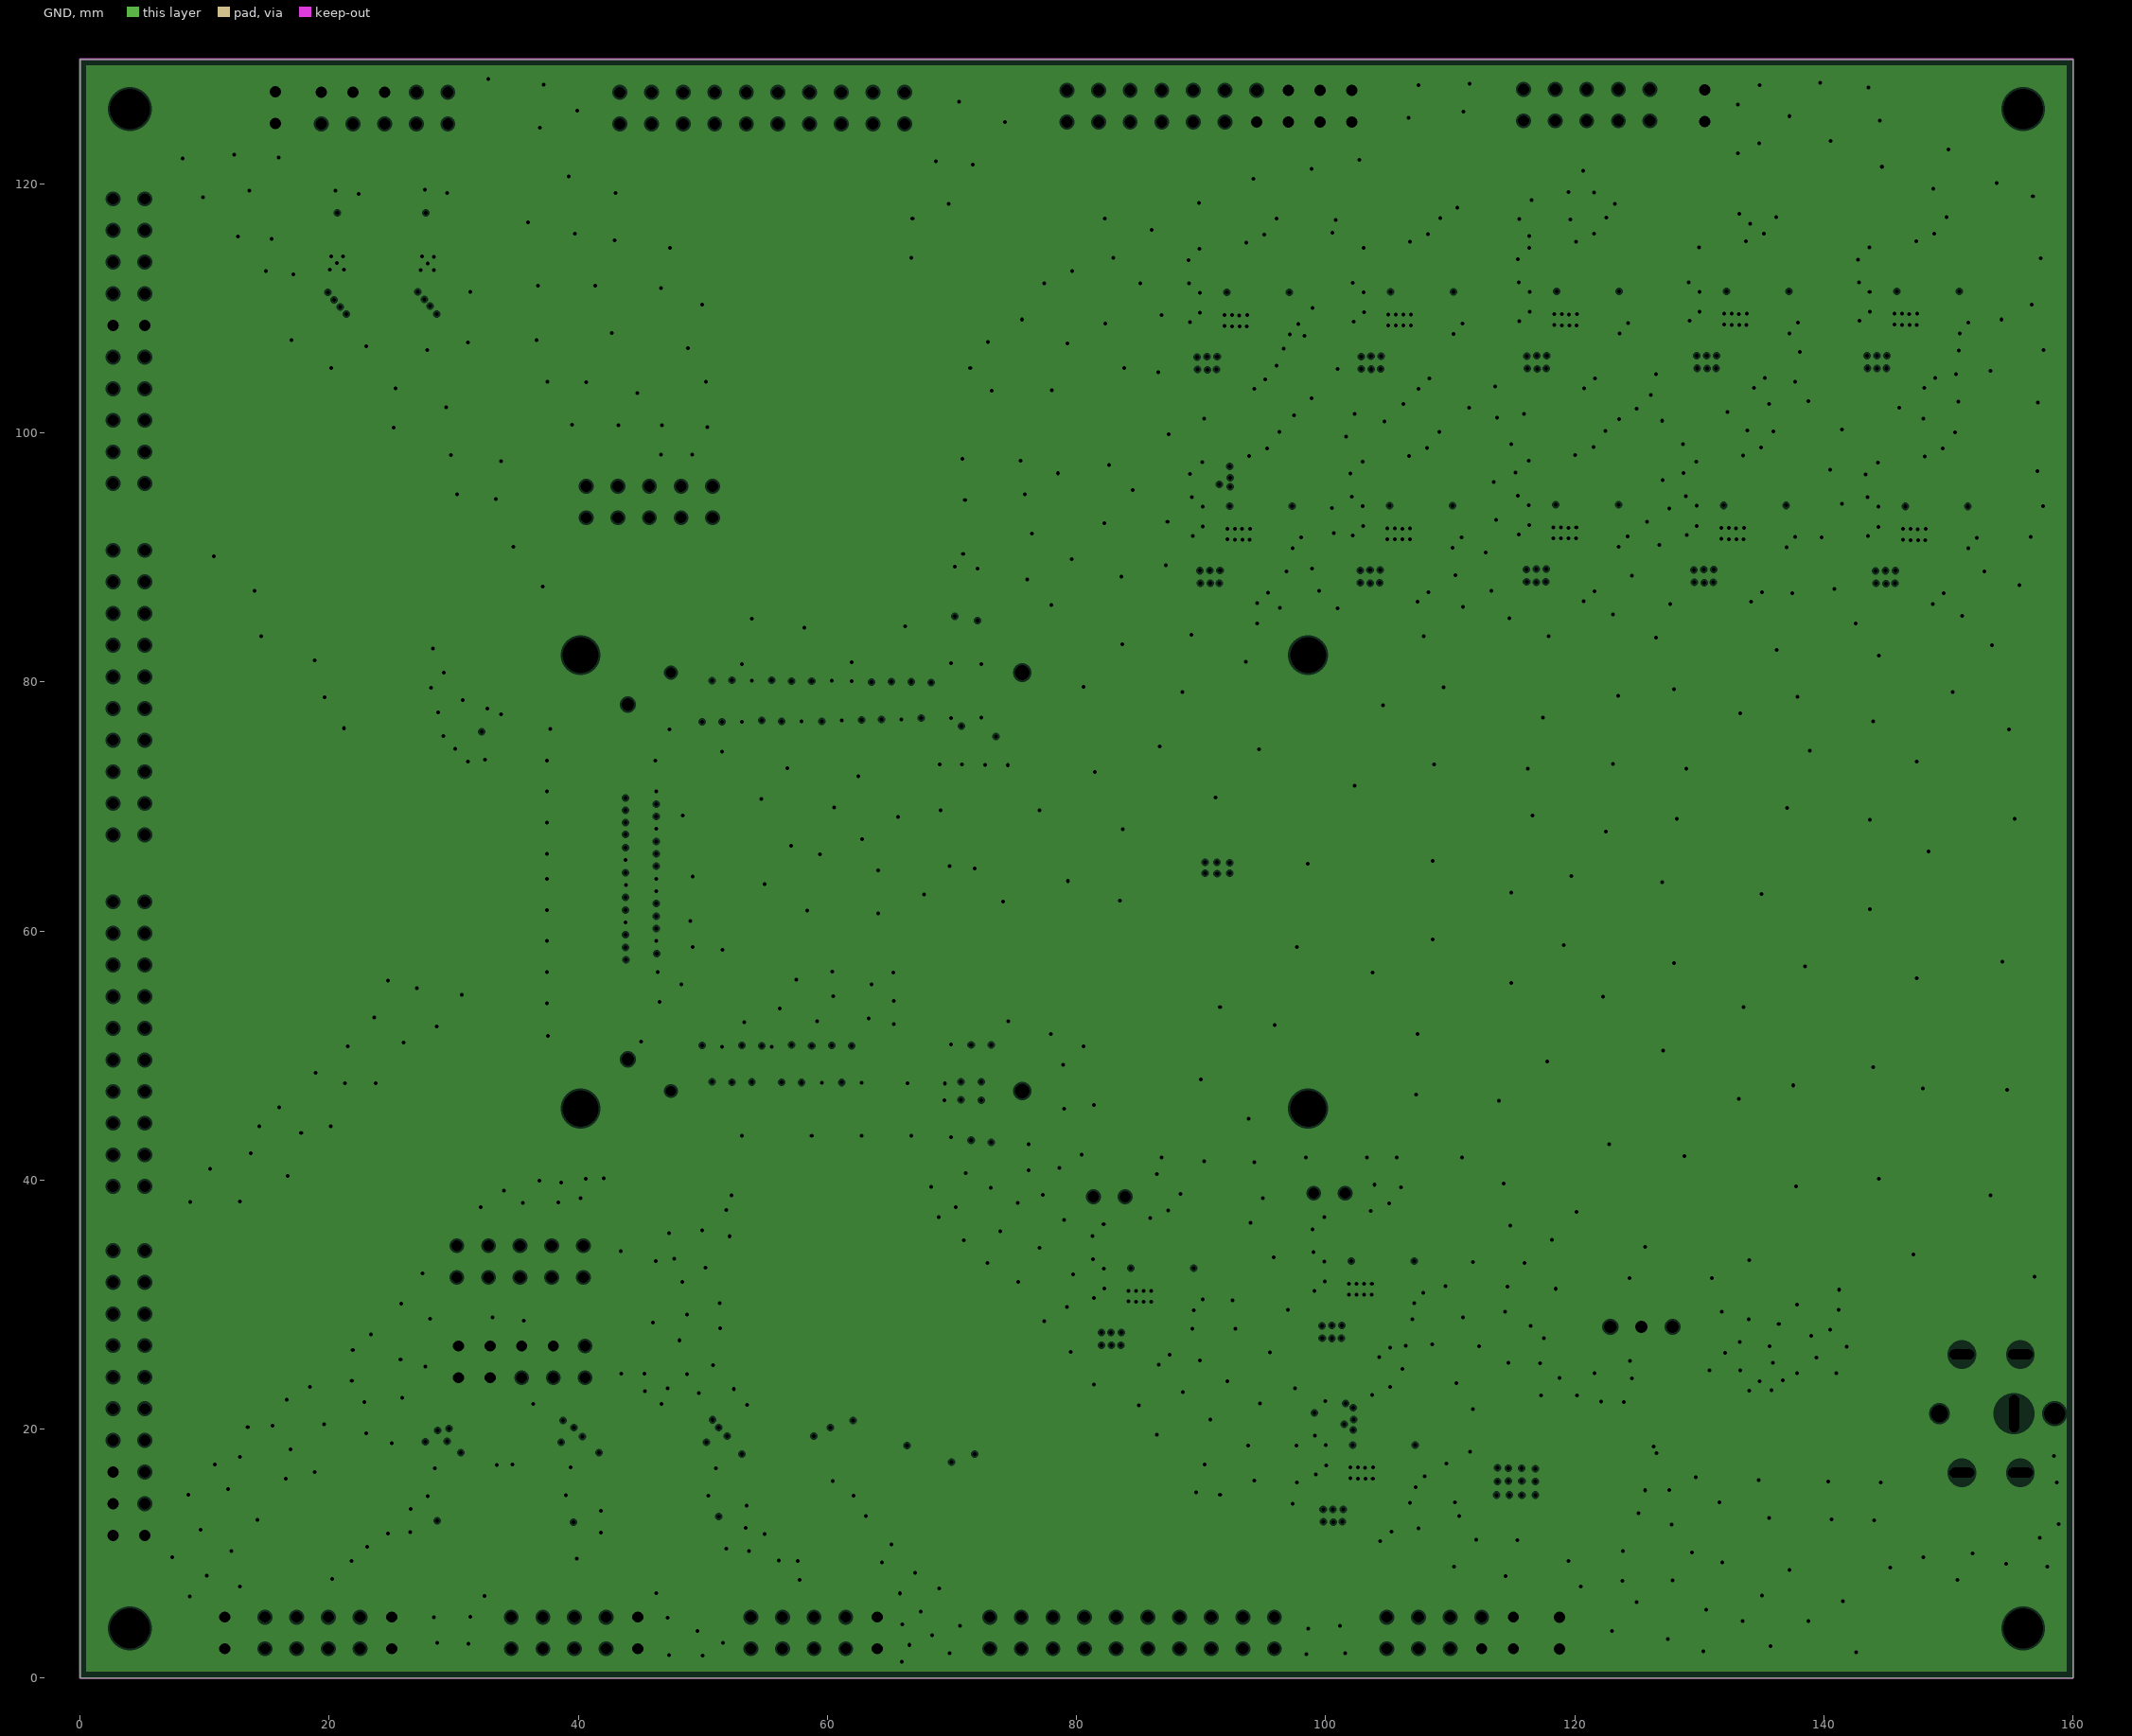
[diagram p0: GND, clearances drawn from the general rule]
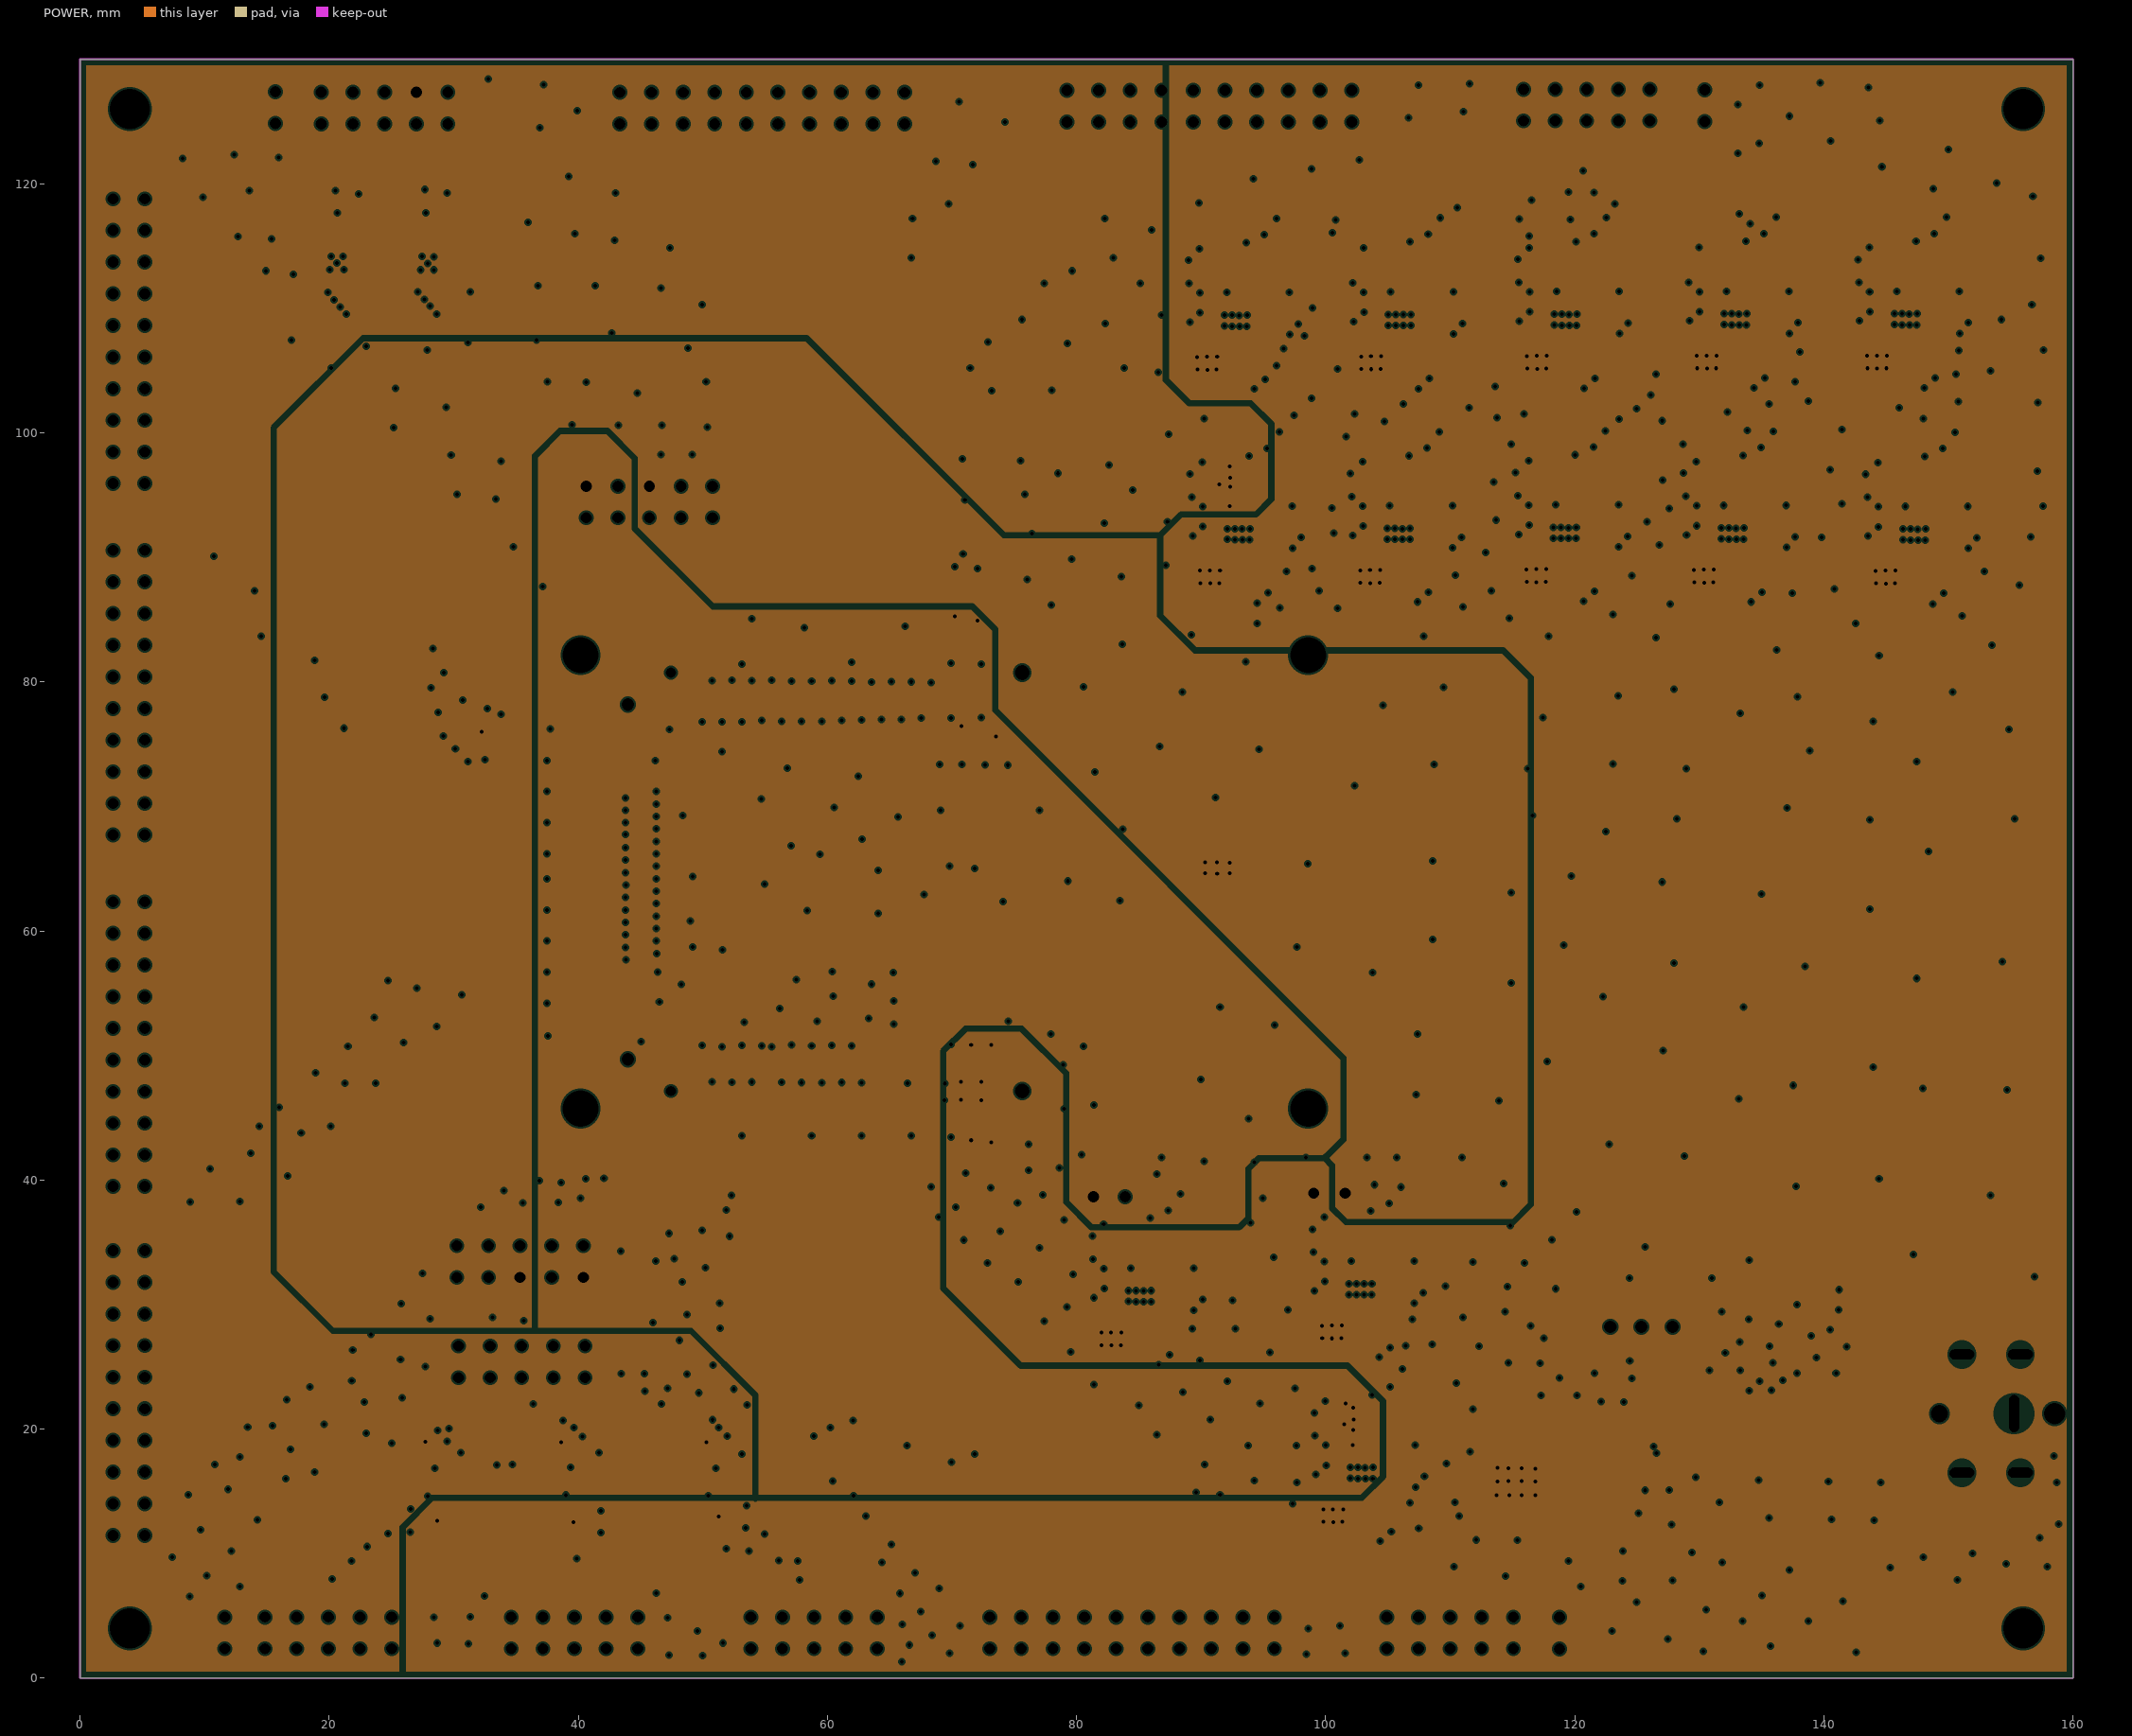
[diagram p1: POWER, clearances drawn from the general rule]
# Altium PCB MISC82195.PcbDoc (part 2 of 8)
## Components (designator, comment, footprint, x,y, rotation, side; value= is the part's Value field where it differs from the comment) (continued)
VR9 "50kΩ" RES-ADJ-SMD_3224W 110.381,97.333 r180 top
VR10 "50kΩ" RES-ADJ-SMD_3224W 107.417,36.652 r180 top
VR11 "50kΩ" RES-ADJ-SMD_3224W 89.603,36.119 r180 top
VR12 "50kΩ" RES-ADJ-SMD_3224W 107.409,21.92 r180 top
VR13 "50kΩ" RES-ADJ-SMD_3224W 97.528,97.307 r180 top

## Footprints (in the part's own frame and the unit in brackets; to place one, negate y for a bottom-side part, rotate by r counter-clockwise, add the part's x,y. Pads: shape width x height; smd on the part's side, far side on the other; paste and mask are expansions set on the pad)
3225-6p [mm]
  rect 1.05x1 smd: 1(-1.125,-0.8) 3(1.125,-0.8) 4(1.125,0.8) 6(-1.125,0.8)
  rect 0.65x1 smd: 2(0,-0.8) 5(0,0.8)
  silkscreen extent -1.6,-1.79 1.6,0.22
C0603 [mm]
  rect 0.8x0.9 smd: 1(-0.7,0) 2(0.7,0)
  silkscreen extent -1.41,-0.71 1.39,0.72
DC-IN-TH_HX-DC007B-2.5 [mm]
  round 1.7 hole 1.7 unplated: 0(-6,0)
  round 2.2 hole 1.4: 1(3.25,0)
  oval 1.4x3.8 hole 0.8 slot 3 at 90 deg: 2(-2.75,0)
  oval 2.8x1.4 hole 0.8 slot 2 at 0 deg: 3(-3.25,4.75) 3(-3.25,-4.75) 3(1.45,4.75) 3(1.45,-4.75)
  silkscreen extent -8.75,-5 4.25,5
DFN-10_L3.0-W3.0-P0.50-BL-EP-3 [mm]
  rect 0.25x0.65 smd: 1(-1,-1.411) 2(-0.5,-1.411) 3(0,-1.411) 4(0.5,-1.411) 5(1,-1.411) 6(1,1.411) 7(0.5,1.411) 8(0,1.411) 9(-0.5,1.411) 10(-1,1.411)
  rect 2.5x1.6 smd: 11(0,0)
  silkscreen extent -1.58,-2 1.58,1.58
FILTER-SMD_4P-L7.0-W6.0-TL_SMCM7060 [mm]
  rect 2.5x1.75 smd: 1(-2.75,1.625) 2(-2.75,-1.625) 3(2.75,-1.625) 4(2.75,1.625)
  silkscreen extent -3.94,-3.05 3.94,3.05
HDR2.54-LI-2P [mm] "排针，2脚"
  rect 1.7x1.7 hole 0.9: 1(-1.27,0)
  round 1.7 hole 0.9: 2(1.27,0)
  silkscreen extent -2.54,-1.27 2.54,1.27, body extent -2.54,-1.27 2.54,1.27, height 2.54
HDR2.54-LI-2x5P [mm] "双排排针，5x2脚"
  rect 1.6x1.6 hole 0.9: 1(-5.08,-1.27)
  round 1.6 hole 0.9: 2(-5.08,1.27) 3(-2.54,-1.27) 4(-2.54,1.27) 5(0,-1.27) 6(0,1.27) 7(2.54,-1.27) 8(2.54,1.27) 9(5.08,-1.27) 10(5.08,1.27)
  silkscreen extent -6.35,-2.54 6.35,2.54, body extent -6.35,-2.54 6.35,2.54, height 8.5
HDR2.54-LI-2x10P [mm] "双排排针，10x2脚"
  rect 1.6x1.6 hole 0.9: 1(-11.43,-1.27)
  round 1.6 hole 0.9: 2(-11.43,1.27) 3(-8.89,-1.27) 4(-8.89,1.27) 5(-6.35,-1.27) 6(-6.35,1.27) 7(-3.81,-1.27) 8(-3.81,1.27) 9(-1.27,-1.27) 10(-1.27,1.27) 11(1.27,-1.27) 12(1.27,1.27) 13(3.81,-1.27) 14(3.81,1.27) 15(6.35,-1.27) 16(6.35,1.27) 17(8.89,-1.27) 18(8.89,1.27) 19(11.43,-1.27) 20(11.43,1.27)
  silkscreen extent -12.7,-2.54 12.7,2.54, body extent -12.7,-2.54 12.7,2.54, height 8.5
LED0805-R-RD [mm]
  rect 1x1.4 smd: 1(1.05,0) 2(-1.05,0)
  silkscreen extent -2.22,-1.04 1.99,1.01
M2.9 [mm]
  round 4.2 hole 2.9: 1(15.421,1.401)
M3 [mm]
  round 6 hole 3.2: 1(0.004,-0.002)
R0603 [mm]
  rect 0.806x0.864 smd paste-100 mask+0.051: 1(-0.753,0) 2(0.753,0)
  silkscreen extent -1.39,-0.66 1.39,0.66
RES-ADJ-SMD_3224W [mm]
  rect 1.3x2 smd: 1(-1.25,-1.45) 3(1.25,-1.45)
  rect 2x1.6 smd: 2(0,1.45)
  silkscreen extent -2.36,-3.36 2.47,1.77
SMA_L4.2-W2.7-LS5.0-BI [mm]
  rect 2x1.8 smd: 1(-2,0) 2(2,0)
  silkscreen extent -2.3,-1.4 2.3,1.4
SMB_L4.6-W3.6-LS5.3-RD [mm]
  rect 2.047x2.192 smd: 1(-2.361,0) 2(2.361,0)
  silkscreen extent -3.12,-1.96 2.74,1.96
SW-SMD_4P-L6.0-W6.0-P4.50-LS9.0-2 [mm]
  rect 2.3x1.5 smd: 1(-4.55,2.25) 2(4.55,2.25) 3(-4.55,-2.25) 4(4.55,-2.25)
  silkscreen extent -3,-3 3,3
SW-TH_K3-1204D [mm]
  round 1.5 hole 1: 1(-2.5,0) 2(0,0) 3(2.5,0)
  silkscreen extent -5,-1.25 5,1.25
VQFN-10_L2.0-W2.0-P0.45-TL [mm]
  round 0.6 smd: 1(-0.915,0.9) 4(-0.905,-0.9) 7(0.915,-0.9) 10(0.915,0.9)
  rect 0.6x0.25 smd paste+0 mask+0.05: 2(-0.905,0.225) 3(-0.905,-0.225) 8(0.905,-0.225) 9(0.905,0.225)
  rect 0.3x2.4 smd paste+0 mask+0.05: 5(-0.235,0) 6(0.265,0)
  Top Layer region: -0.865,1.2 -0.865,0.9 -1.215,0.9 -1.215,0.6 -0.615,0.6 -0.615,0.9 -0.615,0.9 -0.615,1.2
  Top Layer region: -0.855,-1.2 -0.855,-0.9 -1.205,-0.9 -1.205,-0.6 -0.605,-0.6 -0.605,-0.9 -0.605,-0.9 -0.605,-1.2
  Top Layer region: 0.865,-1.2 0.865,-0.9 1.215,-0.9 1.215,-0.6 0.615,-0.6 0.615,-0.9 0.615,-0.9 0.615,-1.2
  Top Layer region: 0.865,1.2 0.865,0.9 1.215,0.9 1.215,0.6 0.615,0.6 0.615,0.9 0.615,0.9 0.615,1.2
  silkscreen extent -1.85,-1.28 1.34,1.36
WQFN-16(3x3) [mm]
  oval 0.6x0.24 smd mask+0.05: 1(-1.4,0.75) 2(-1.4,0.25) 3(-1.4,-0.25) 4(-1.4,-0.75) 9(1.4,-0.75) 10(1.4,-0.25) 11(1.4,0.25) 12(1.4,0.75)
  oval 0.24x0.6 smd mask+0.05: 5(-0.75,-1.4) 6(-0.25,-1.4) 7(0.25,-1.4) 8(0.75,-1.4) 13(0.75,1.4) 14(0.25,1.4) 15(-0.25,1.4) 16(-0.75,1.4)
  rect 1.68x1.68 smd: 17(0,0)
  silkscreen extent -2.38,-1.72 1.72,1.72
WQFN-16_L3.0-W3.0-P0.50-BL-EP0.8 [mm]
  rect 0.28x0.665 smd: 1(-0.75,-1.407) 2(-0.25,-1.407) 3(0.25,-1.407) 4(0.75,-1.407) 9(0.75,1.407) 10(0.25,1.407) 11(-0.25,1.407) 12(-0.75,1.407)
  rect 0.665x0.28 smd: 5(1.407,-0.75) 6(1.407,-0.25) 7(1.407,0.25) 8(1.407,0.75) 13(-1.407,0.75) 14(-1.407,0.25) 15(-1.407,-0.25) 16(-1.407,-0.75)
  rect 0.8x0.8 smd: 17(0,0)
  silkscreen extent -1.58,-2 1.58,1.58
XMS6302-A [mm]
  rect 0.5x2 smd mask+0.1: A1(-11.6,2.2) A2(-11.6,-2.2) A3(-10.8,2.2) A4(-10.8,-2.2) A5(-10,2.2) A6(-10,-2.2) A7(-9.2,2.2) A8(-9.2,-2.2) A9(-8.4,2.2) A10(-8.4,-2.2) A11(-7.6,2.2) A12(-7.6,-2.2) A13(-6.8,2.2) A14(-6.8,-2.2) A15(-6,2.2) A16(-6,-2.2) A17(-5.2,2.2) A18(-5.2,-2.2) A19(-4.4,2.2) A20(-4.4,-2.2) A21(-3.6,2.2) A22(-3.6,-2.2) A23(-2.8,2.2) A24(-2.8,-2.2) A25(-2,2.2) A26(-2,-2.2) A27(-1.2,2.2) A28(-1.2,-2.2) A29(-0.4,2.2) A30(-0.4,-2.2) A31(0.4,2.2) A32(0.4,-2.2) A33(1.2,2.2) A34(1.2,-2.2) A35(2,2.2) A36(2,-2.2) A37(2.8,2.2) A38(2.8,-2.2) A39(3.6,2.2) A40(3.6,-2.2) A41(4.4,2.2) A42(4.4,-2.2) A43(5.2,2.2) A44(5.2,-2.2) A45(6,2.2) A46(6,-2.2) A47(6.8,2.2) A48(6.8,-2.2) A49(7.6,2.2) A50(7.6,-2.2) A51(8.4,2.2) A52(8.4,-2.2) A53(9.2,2.2) A54(9.2,-2.2) A55(10,2.2) A56(10,-2.2) A57(10.8,2.2) A58(10.8,-2.2) A59(11.6,2.2) A60(11.6,-2.2)
  round 0.8 hole 0.8 unplated: ""(-14.1,0)
  round 1.2 hole 1.2 unplated: ""(14.1,0)
  silkscreen extent -14.9,-3 14.9,4.04
XMS6302-B [mm]
  rect 0.305x1.448 smd mask+0.05: B1(-12.25,3.086) B2(-12.25,-3.086) B3(-11.75,3.086) B4(-11.75,-3.086) B5(-11.25,3.086) B6(-11.25,-3.086) B7(-10.75,3.086) B8(-10.75,-3.086) B9(-10.25,3.086) B10(-10.25,-3.086) B11(-9.75,3.086) B12(-9.75,-3.086) B13(-9.25,3.086) B14(-9.25,-3.086) B15(-8.75,3.086) B16(-8.75,-3.086) B17(-8.25,3.086) B18(-8.25,-3.086) B19(-7.75,3.086) B20(-7.75,-3.086) B21(-7.25,3.086) B22(-7.25,-3.086) B23(-6.75,3.086) B24(-6.75,-3.086) B25(-6.25,3.086) B26(-6.25,-3.086) B27(-5.75,3.086) B28(-5.75,-3.086) B29(-5.25,3.086) B30(-5.25,-3.086) B31(-4.75,3.086) B32(-4.75,-3.086) B33(-4.25,3.086) B34(-4.25,-3.086) B35(-3.75,3.086) B36(-3.75,-3.086) B37(-3.25,3.086) B38(-3.25,-3.086) B39(-2.75,3.086) B40(-2.75,-3.086) B41(-2.25,3.086) B42(-2.25,-3.086) B43(-1.75,3.086) B44(-1.75,-3.086) B45(-1.25,3.086) B46(-1.25,-3.086) B47(-0.75,3.086) B48(-0.75,-3.086) B49(-0.25,3.086) B50(-0.25,-3.086) B51(0.25,3.086) B52(0.25,-3.086) B53(0.75,3.086) B54(0.75,-3.086) B55(1.25,3.086) B56(1.25,-3.086) B57(1.75,3.086) B58(1.75,-3.086) B59(2.25,3.086) B60(2.25,-3.086) B61(2.75,3.086) B62(2.75,-3.086) B63(3.25,3.086) B64(3.25,-3.086) B65(3.75,3.086) B66(3.75,-3.086) B67(4.25,3.086) B68(4.25,-3.086) B69(4.75,3.086) B70(4.75,-3.086) B71(5.25,3.086) B72(5.25,-3.086) B73(5.75,3.086) B74(5.75,-3.086) B75(6.25,3.086) B76(6.25,-3.086) B77(6.75,3.086) B78(6.75,-3.086) B79(7.25,3.086) B80(7.25,-3.086) B81(7.75,3.086) B82(7.75,-3.086) B83(8.25,3.086) B84(8.25,-3.086) B85(8.75,3.086) B86(8.75,-3.086) B87(9.25,3.086) B88(9.25,-3.086) B89(9.75,3.086) B90(9.75,-3.086) B91(10.25,3.086) B92(10.25,-3.086) B93(10.75,3.086) B94(10.75,-3.086) B95(11.25,3.086) B96(11.25,-3.086) B97(11.75,3.086) B98(11.75,-3.086) B99(12.25,3.086) B100(12.25,-3.086)
  round 1.016 hole 1.016 unplated: ""(-14.238,2.032) ""(14.238,2.032)
  silkscreen extent -15,-2.99 15,4.17
XMS6302-C [mm]
  rect 0.5x2 smd mask+0.1: C1(-11.6,2.2) C2(-11.6,-2.2) C3(-10.8,2.2) C4(-10.8,-2.2) C5(-10,2.2) C6(-10,-2.2) C7(-9.2,2.2) C8(-9.2,-2.2) C9(-8.4,2.2) C10(-8.4,-2.2) C11(-7.6,2.2) C12(-7.6,-2.2) C13(-6.8,2.2) C14(-6.8,-2.2) C15(-6,2.2) C16(-6,-2.2) C17(-5.2,2.2) C18(-5.2,-2.2) C19(-4.4,2.2) C20(-4.4,-2.2) C21(-3.6,2.2) C22(-3.6,-2.2) C23(-2.8,2.2) C24(-2.8,-2.2) C25(-2,2.2) C26(-2,-2.2) C27(-1.2,2.2) C28(-1.2,-2.2) C29(-0.4,2.2) C30(-0.4,-2.2) C31(0.4,2.2) C32(0.4,-2.2) C33(1.2,2.2) C34(1.2,-2.2) C35(2,2.2) C36(2,-2.2) C37(2.8,2.2) C38(2.8,-2.2) C39(3.6,2.2) C40(3.6,-2.2) C41(4.4,2.2) C42(4.4,-2.2) C43(5.2,2.2) C44(5.2,-2.2) C45(6,2.2) C46(6,-2.2) C47(6.8,2.2) C48(6.8,-2.2) C49(7.6,2.2) C50(7.6,-2.2) C51(8.4,2.2) C52(8.4,-2.2) C53(9.2,2.2) C54(9.2,-2.2) C55(10,2.2) C56(10,-2.2) C57(10.8,2.2) C58(10.8,-2.2) C59(11.6,2.2) C60(11.6,-2.2)
  round 0.8 hole 0.8 unplated: ""(-14.1,0)
  round 1.2 hole 1.2 unplated: ""(14.1,0)
  silkscreen extent -14.9,-3 14.9,4.02

## Part data
C1 C2 C3 C4 C5 C6 C7 C9 C10 C11 C12 C13 C14 C15 C16 C17 C18 C19 C20 C21 C22 C23 C24 C25 C26 C27 C28 C29 C30 C31 C32 C33 C34 C35 C36 C37 C38 C39 C40 C41 C42 C43 C44 C45 C46 C47 C48 C49 C50 C51 C52 C53 C54 C61 C62 C65 C66 C68 C69 C70 C71 C72 C73 C74 C75 C76 C77 C78 C79 C80 C81 C82 C83: library part C, "SMD capacitor"
C8: library part CC0603KRX7R9BB104
C55 C56: library part 10nF
C57 C58 C59 C60: library part 1uF
C63 C64: library part CL21A226MAQNNNE
C67: library part CC0603KRX7R9BB103
D3: library part VS-10BQ015HM3/5BT
D4: library part SMAJ12CA_C908818
F1 F2 F3 F4: "Standoff hole"
JP1 JP4 JP8 JP11 JP12 JP13 JP14 JP15 JP16: "5*2P connector"
JP2 JP3 JP5 JP6 JP7 JP9 JP10: library part "Header 10X2", "10*2P connector"
JP17 JP18 JP19 JP20 JP21 JP22: library part "Header 2", "2P connector"
L1: library part ACM7060-301-2PL-TL01
LED1: library part NCD0805G1
M1 M2 M3 M4: library part M2, "SMD standoff"
R1 R2 R3 R4 R5 R6 R7 R8 R9 R10 R11 R12 R13 R14 R15 R16 R17 R18 R19 R20 R21 R22 R23 R24 R25 R26 R27 R28 R29 R30 R31 R32 R33 R34 R35 R36 R37 R38 R42 R43 R44 R45 R46 R47 R48 R49 R50 R51 R52 R53 R54 R55 R56 R57 R58: library part R, "SMD resistor"
R39 R41: library part Res_0603
R40: library part CR0805F681RP05Z
SW1: library part K3-1204D
U1: library part SiT9121AI, "100MHz oscillator"
U2 U3 U4 U5 U6 U7 U8 U9 U10 U16 U17 U18 U19: library part LT3045IDD#PBF
U14: library part TPS259472ARPWR
U15: library part "HX DC007B-2.5"
VR1 VR2 VR3 VR4 VR5 VR6 VR7 VR8 VR9 VR10 VR11 VR12 VR13: library part 3224W-1-503E

## Free pads (board coordinates)
  round 1 smd mask+1: MARK(9.957,126.695) MARK(148.514,127.381) MARK(148.819,2.692)

## Via types
v1: diameter 0.508, hole 0.305, Top Layer to Bottom Layer, 1218 vias

## Nets (pads, with @x,y where several pads share a name; then routed paths per layer and width w, separated by ;. In a path a pad name is that pad's centre, name@x,y a point inside that pad or via, vN(x,y) a via of type N, cw(c..) or ccw(c..) an arc to the next point about the centre after c; other vN are vias at no path point)
CDAC1_OUT0: D1.2 JP14.4 | length 12.7
  Top Layer w0.254: D1.2@26.48,113.874 25.622,113.874 24.74,114.757 24.74,121.183 26.873,123.317 JP14.4@26.873,124.435